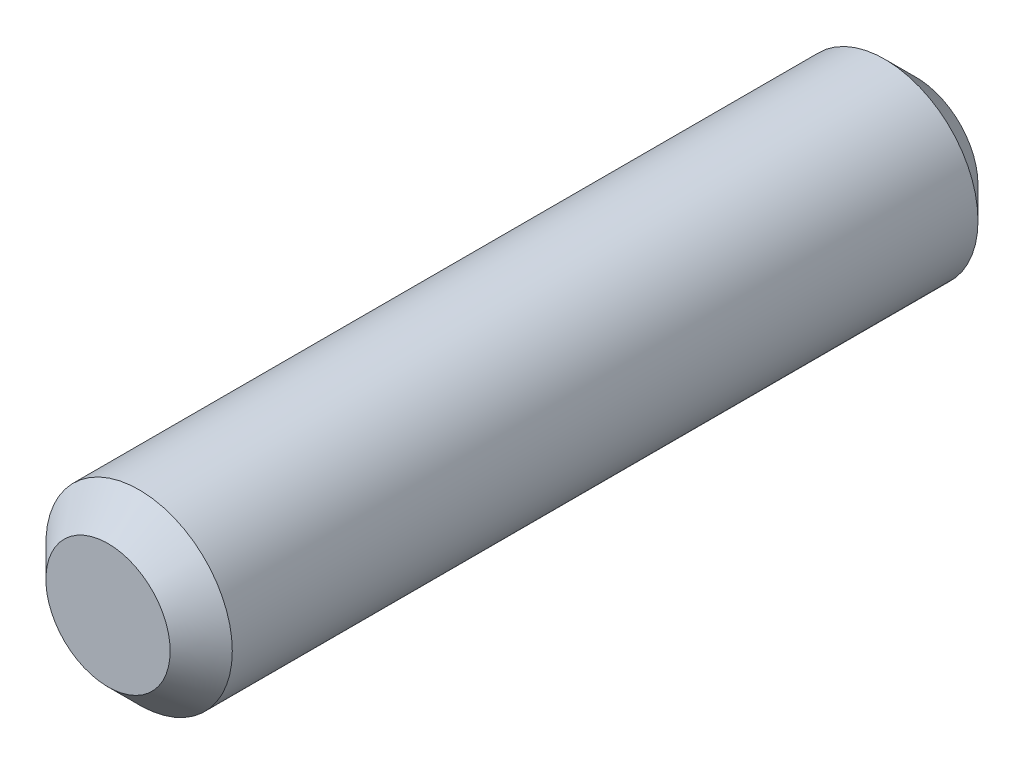
SolidWorks part; units mm, degrees
ref_plane "前视基准面" through (0, 0, 0) normal (0, 0, 1) x (1, 0, 0)
ref_plane "上视基准面" through (0, 0, 0) normal (0, 1, 0) x (1, 0, 0)
ref_plane "右视基准面" through (0, 0, 0) normal (1, 0, 0) x (0, 0, -1)
sketch "草图1" plane through (0, 0, 0) normal (0, 0, 1) x (1, 0, 0)
  circle A0 centre (-185.609, 197.4787) radius 1.5 construction
  circle A1 centre (-185.609, 197.4787) radius 1.5
extrude "凸台-拉伸1" add sketch "草图1" against normal up to surface (13 mm away)
chamfer "倒角1" distance 0.5 angle 45 2 edges at (-184.109, 197.4787, 0) (-185.609, 195.9787, -13)
